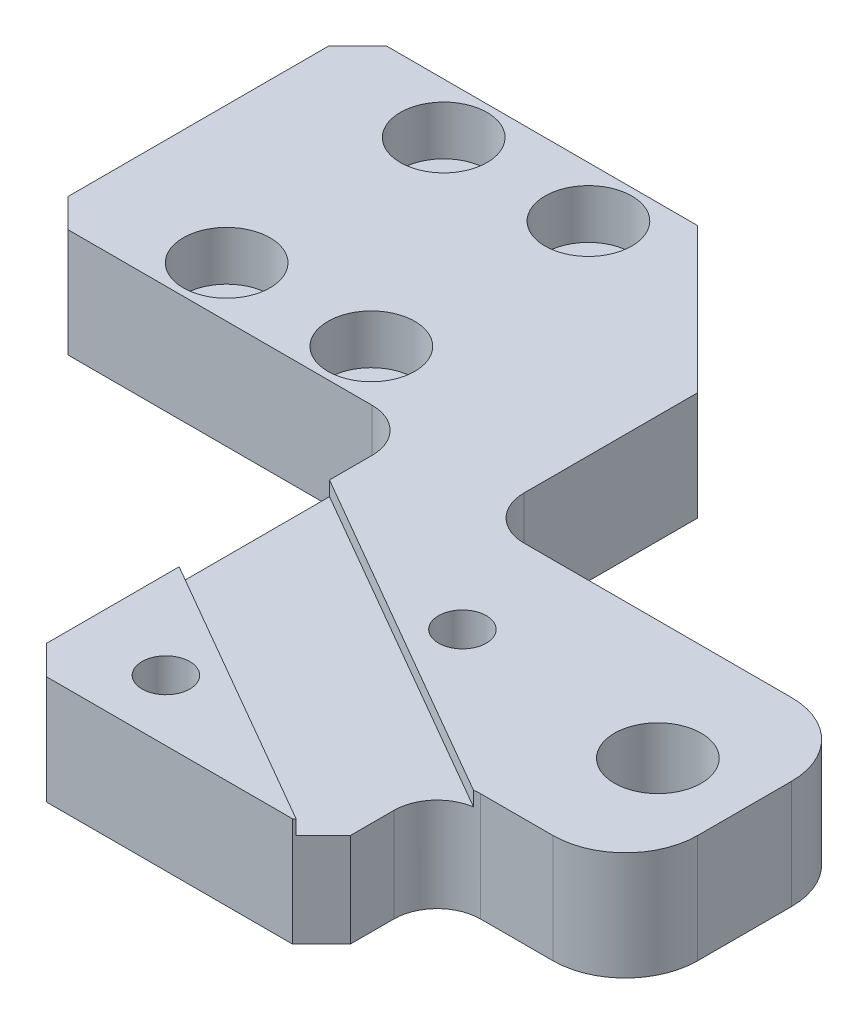
SolidWorks part; units mm, degrees
ref_plane "Front Plane" through (0, 0, 0) normal (0, 0, 1) x (1, 0, 0)
ref_plane "Top Plane" through (0, 0, 0) normal (0, 1, 0) x (1, 0, 0)
ref_plane "Right Plane" through (0, 0, 0) normal (1, 0, 0) x (0, 0, -1)
sketch "Sketch1" plane through (0, 0, 0) normal (0, 1, 0) x (1, 0, 0)
  line L1 (-30, -24.75) -> (30, -24.75)
  line L2 (-30, -24.75) -> (-30, 24.75)
  line L3 (-30, 24.75) -> (30, 24.75)
  line L4 (30, -24.75) -> (30, 24.75)
  line L5 (-30, -24.75) -> (30, 24.75) construction
  line L6 (-30, 24.75) -> (30, -24.75) construction
  point P0 (0, 0)
  dimension "D1" = 49.5
  dimension "D2" = 60
extrude "Boss-Extrude1" add sketch "Sketch1" along normal blind 7.5
sketch "Sketch2" plane through (0, 7.5, 0) normal (0, 1, 0) x (1, 0, 0)
  line L1 (30, 24.75) -> (3.5, 24.75)
  line L2 (30, 24.75) -> (30, -0.25)
  line L3 (30, -0.25) -> (3.5, -0.25)
  line L4 (3.5, 24.75) -> (3.5, -0.25)
  line L5 (30, -24.75) -> (17, -24.75)
  line L6 (30, -24.75) -> (30, -16.75)
  line L7 (30, -16.75) -> (17, -16.75)
  line L8 (17, -24.75) -> (17, -16.75)
  line L9 (-30, -24.75) -> (-4, -24.75)
  line L10 (-30, -24.75) -> (-30, 2.75)
  line L11 (-30, 2.75) -> (-4, 2.75)
  line L12 (-4, -24.75) -> (-4, 2.75)
  dimension "D1" = 25
  dimension "D2" = 26.5
  dimension "D3" = 13
  dimension "D4" = 8
  dimension "D5" = 27.5
  dimension "D6" = 26
extrude "Cut-Extrude1" cut sketch "Sketch2" against normal through all
hole_wizard "Hole wizard: socket head cap screw, type 1" positions "Sketch3" profile "Sketch4" counterbore size "M3" standard "GB" end condition through all
sketch "Sketch3" plane through (0, 7.5, 0) normal (0, 1, 0) x (1, 0, 0)
  line L0 (3.5, 24.75) -> (-30, 24.75) construction
  line L1 (-30, 24.75) -> (-30, 2.75) construction
  line L3 (-10.55, 21.25) -> (-20.55, 21.25) construction
  line L4 (-10.55, 21.25) -> (-10.55, 6.25) construction
  line L5 (-10.55, 6.25) -> (-20.55, 6.25) construction
  line L6 (-20.55, 21.25) -> (-20.55, 6.25) construction
  point P0 (-10.55, 21.25)
  point P52 (-20.55, 21.25)
  point P55 (-20.55, 6.25)
  point P58 (-10.55, 6.25)
  dimension "D1" = 3.5
  dimension "D2" = 19.45
  dimension "D3" = 15
  dimension "D4" = 10
sketch "Sketch4" plane through (-10.55, 7.5, -21.25) normal (1, 0, 0) x (0, 0, 1)
  line L0 (0, 0) -> (0, 7.5)
  line L1 (0, 7.5) -> (1.7, 7.5)
  line L3 (1.7, 7.5) -> (1.7, 3.4)
  line L4 (1.7, 3.4) -> (3, 3.4)
  line L5 (3, 3.4) -> (3, 0)
  line L7 (3, 0) -> (0, 0)
  line L11 (0, -6.35) -> (0, 107.95) construction
  dimension "通孔孔直径" = 3.4
  dimension "通孔孔深度" = 7.5
  dimension "柱形沉头孔直径" = 6
  dimension "柱形沉头孔深度" = 3.4
hole_wizard "Ø6.0 (6) Diameter Hole1" positions "Sketch5" profile "Sketch6" hole size "Ø6.0" standard "GB" end condition through all
sketch "Sketch5" plane through (0, 7.5, 0) normal (0, 1, 0) x (1, 0, 0)
  line L0 (30, -16.75) -> (30, -0.25) construction
  line L1 (24, -0.25) -> (24, -16.75) construction
  line L2 (3.5, -0.25) -> (30, -0.25) construction
  line L3 (30, -16.75) -> (17, -16.75) construction
  point P0 (24, -8.5)
  dimension "D1" = 6
sketch "Sketch6" plane through (24, 7.5, 8.5) normal (1, 0, 0) x (0, 0, 1)
  line L0 (0, 0) -> (0, 7.5)
  line L1 (0, 7.5) -> (3, 7.5)
  line L2 (3, 7.5) -> (3, 0)
  line L5 (3, 0) -> (0, 0)
  line L11 (0, -6.35) -> (0, 107.95) construction
  dimension "通孔孔直径" = 6
  dimension "通孔孔深度" = 7.5
sketch "Sketch7" plane through (0, 7.5, 0) normal (0, 1, 0) x (1, 0, 0)
  line L0 (-12.304, -8.7906) -> (20.3028, -27.6162)
  line L1 (-12.304, -8.7906) -> (-7.804, -0.9964)
  line L2 (20.3028, -27.6162) -> (24.8028, -19.8219)
  line L3 (-7.804, -0.9964) -> (24.8028, -19.8219)
  line L4 (-4, -24.75) -> (-4, 2.75) construction
  dimension "D1" = 60
  dimension "D2" = 9
extrude "Cut-Extrude2" cut sketch "Sketch7" against normal blind 1
fillet "Fillet1" radius 5 2 edges at (30, 3.75, 0.25) (30, 3.75, 16.75)
chamfer "Chamfer1" distance 10 angle 45 1 edges at (3.5, 3.75, -24.75)
chamfer "Chamfer2" distance 2 angle 45 4 edges at (17, 3.25, 24.75) (-4, 3.75, 24.75) (-30, 3.75, -2.75) (-30, 3.75, -24.75)
fillet "Fillet2" radius 3 3 edges at (3.5, 3.75, 0.25) (17, 3.25, 16.75) (-4, 3.75, -2.75)
hole_wizard "M4 Tapped Hole1" positions "Sketch8" profile "Sketch9" tap size "M4" standard "GB" end condition through all
sketch "Sketch8" plane through (0, 7.5, 0) normal (0, 1, 0) x (1, 0, 0)
  line L0 (-4, -8.3888) -> (17, -20.5132) construction
  line L1 (-4, -13.585) -> (-4, -3.1927) construction
  line L2 (17, -19.75) -> (17, -22.75) construction
  line L4 (19.5427, -16.7851) -> (-4, -3.1927) construction
  line L5 (-4, -13.585) -> (15.1239, -24.6261) construction
  point P0 (9.5386, -7.5451)
  point P2 (2.0386, -20.5354)
  dimension "D1" = 15
sketch "Sketch9" plane through (9.5386, 7.5, 7.5451) normal (1, 0, 0) x (0, 0, 1)
  line L0 (0, 0) -> (0, 7.5)
  line L1 (0, 7.5) -> (1.65, 7.5)
  line L2 (1.65, 7.5) -> (1.65, 0)
  line L5 (1.65, 0) -> (0, 0)
  line L11 (0, -6.35) -> (0, 107.95) construction
  dimension "通孔螺纹孔钻头直径" = 3.3
  dimension "通孔螺纹孔钻头深度" = 7.5
cosmetic thread "Cosmetic thread 1" parameters "D2"=4
cosmetic thread "Cosmetic thread 2" parameters "D2"=4
sketch "Sketch10" plane through (-30, 0, 0) normal (-1, 0, 0) x (0, 0, 1)
  line L0 (-13.75, 7.5) -> (-13.75, 0) construction
  line L2 (-22.75, 7.5) -> (-4.75, 7.5) construction
  line L3 (-22.75, 0) -> (-4.75, 0) construction
  circle A0 centre (-13.75, 3.75) radius 2.75
  dimension "D1" = 5.5
extrude "Cut-Extrude3" cut sketch "Sketch10" against normal blind 8
